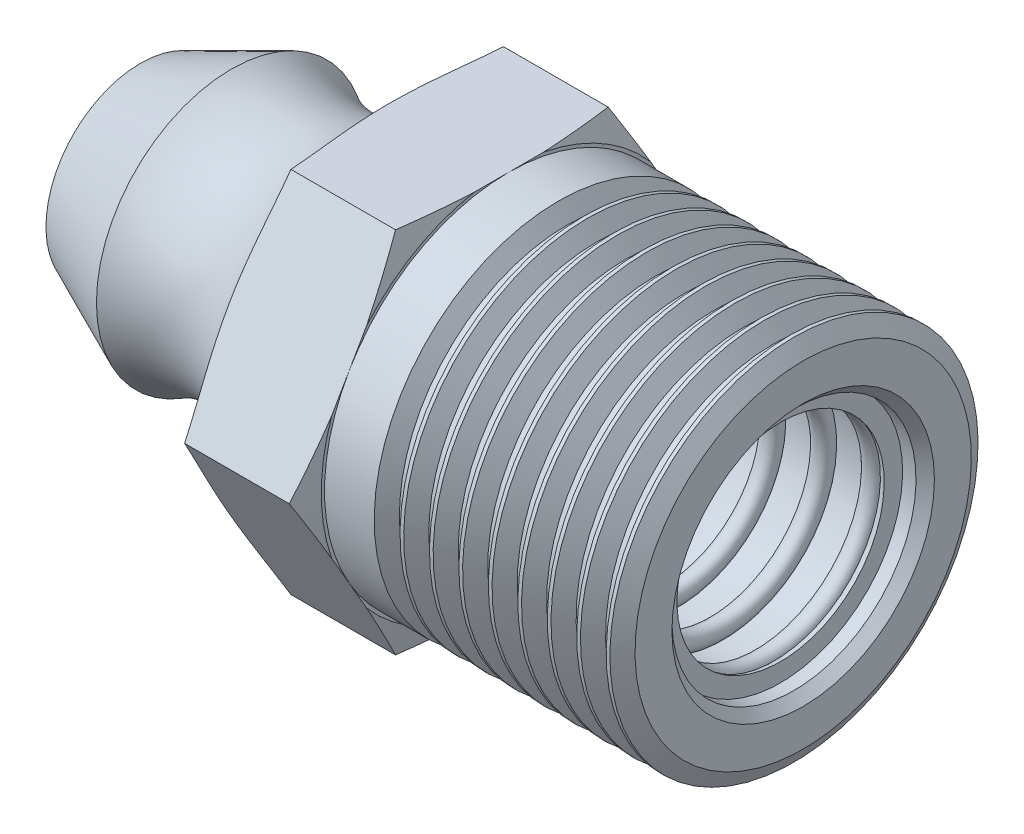
SolidWorks part; units mm, degrees
material "ASTM A36 钢"
ref_plane "前视基准面" through (0, 0, 0) normal (0, 0, 1) x (1, 0, 0)
ref_plane "上视基准面" through (0, 0, 0) normal (0, 1, 0) x (1, 0, 0)
ref_plane "右视基准面" through (0, 0, 0) normal (1, 0, 0) x (0, 0, -1)
sketch "草图1" plane through (0, 0, 0) normal (0, 0, 1) x (1, 0, 0)
  line L0 (-18.4, 0) -> (-15.9, 0)
  line L1 (-8, 5) -> (-8, 5.0885)
  line L2 (-11.5, 2.315) -> (-16.4719, 2.315)
  line L3 (-18, 1.0037) -> (-17.895, 1.0037)
  line L4 (-16.4719, 2.315) -> (-17.895, 1.0037)
  line L5 (-18, 2.565) -> (-15.5294, 3.665)
  line L6 (-0.25, 3.315) -> (-0.6135, 3.315)
  line L7 (-18, 2.565) -> (-18, 1.0037)
  line L8 (-11, 6.0885) -> (-8.2679, 6.0885)
  line L9 (-0.6135, 3.315) -> (-0.6135, 2.815)
  line L11 (-8, 5.0885) -> (-8.2679, 6.0885)
  line L12 (-10.5, 3.315) -> (-11.5, 2.315)
  line L13 (0, 3.565) -> (-0.25, 3.315)
  line L14 (-1.1135, 3.315) -> (-10.5, 3.315)
  line L68 (-6.2, 4.567) -> (-5.95, 5)
  line L69 (-3.2, 4.567) -> (-3, 4.567)
  line L71 (-5.6, 4.567) -> (-5.4, 4.567)
  line L72 (-5.15, 5) -> (-5.05, 5)
  line L73 (-4.35, 5) -> (-4.25, 5)
  line L78 (-6.4, 4.567) -> (-6.2, 4.567)
  line L79 (-5.85, 5) -> (-5.6, 4.567)
  line L80 (-0.8, 4.567) -> (-0.6, 4.567)
  line L81 (-0.25, 5) -> (0, 4.567)
  line L85 (-1.15, 5) -> (-1.05, 5)
  line L90 (-5.95, 5) -> (-5.85, 5)
  line L91 (-5.05, 5) -> (-4.8, 4.567)
  line L92 (-3.45, 5) -> (-3.2, 4.567)
  line L93 (-2.2, 4.567) -> (-1.95, 5)
  line L94 (-1.95, 5) -> (-1.85, 5)
  line L95 (-0.6, 4.567) -> (-0.35, 5)
  line L98 (-1.05, 5) -> (-0.8, 4.567)
  line L102 (-6.65, 5) -> (-6.4, 4.567)
  line L106 (-3.55, 5) -> (-3.45, 5)
  line L112 (-1.85, 5) -> (-1.6, 4.567)
  line L115 (-1.4, 4.567) -> (-1.15, 5)
  line L118 (-3.8, 4.567) -> (-3.55, 5)
  line L119 (-1.6, 4.567) -> (-1.4, 4.567)
  line L125 (-4.8, 4.567) -> (-4.6, 4.567)
  line L126 (-2.75, 5) -> (-2.65, 5)
  line L127 (-8, 5) -> (-6.65, 5)
  line L128 (-4, 4.567) -> (-3.8, 4.567)
  line L134 (-5.4, 4.567) -> (-5.15, 5)
  line L135 (-3, 4.567) -> (-2.75, 5)
  line L136 (-0.35, 5) -> (-0.25, 5)
  line L139 (-4.25, 5) -> (-4, 4.567)
  line L140 (-2.65, 5) -> (-2.4, 4.567)
  line L143 (-4.6, 4.567) -> (-4.35, 5)
  line L144 (-2.4, 4.567) -> (-2.2, 4.567)
  line L171 (0, 0) -> (-15.9, 0) construction
  line L178 (0, 4.567) -> (0, 3.565)
  circle A0 centre (-2.3502, 2.9066) radius 0.25
  arc A1 (-11, 6.0885) -> (-15.5294, 3.665) centre (-13.9601, 6.1764) cw
  arc A2 (-0.8635, 3.065) -> (-0.6135, 2.815) centre (-0.6135, 3.065) ccw
  arc A3 (-15.9, 0) -> (-18.4, 0) centre (-17.15, 0) ccw
  arc A4 (-0.8635, 3.065) -> (-1.1135, 3.315) centre (-1.1135, 3.065) ccw
  circle A5 centre (-1.1194, 3.0577) radius 0.25
  circle A6 centre (-3.581, 2.7555) radius 0.25
  circle A7 centre (-4.8117, 2.6043) radius 0.25
  circle A8 centre (-6.0425, 2.4532) radius 0.25
  circle A9 centre (-7.2732, 2.3021) radius 0.25
  circle A10 centre (-8.504, 2.151) radius 0.25
  circle A11 centre (-9.7347, 1.9999) radius 0.25
  circle A12 centre (-10.9655, 1.8488) radius 0.25
  circle A13 centre (-12.1963, 1.6976) radius 0.25
  circle A14 centre (-13.427, 1.5465) radius 0.25
  circle A15 centre (-14.6578, 1.3954) radius 0.25
  circle A16 centre (-15.8885, 1.2443) radius 0.25
  point P92 (-8, 6.0885)
  point P94 (-8, 6.0885)
  point P95 (0, 3.315)
  dimension "D4" = 45
  dimension "D5" = 5
  dimension "D6" = 0.5
  dimension "D8" = 1.25
  dimension "D9" = 0.35
  dimension "D1" = 1
  dimension "D7" = 2.9614
  dimension "D2" = 15
  dimension "D3" = 0.25
  dimension "D10" = 0.8
  dimension "D11" = 8
  dimension "D12" = 0.8635
  dimension "D13" = 1.2443
  dimension "D14" = 1.1194
  dimension "D15" = 1.3954
  dimension "D16" = 1.5465
  dimension "D17" = 1.6976
  dimension "D18" = 1.8488
  dimension "D19" = 1.9999
  dimension "D20" = 2.151
  dimension "D21" = 2.3502
  dimension "D22" = 2.3021
  dimension "D23" = 2.315
  dimension "D24" = 2.4532
  dimension "D25" = 2.565
  dimension "D26" = 2.6043
  dimension "D27" = 2.7555
  dimension "D28" = 2.815
  dimension "D29" = 3.581
  dimension "D30" = 2.9066
  dimension "D31" = 3.0577
  dimension "D32" = 3.665
  dimension "D36" = 4.8117
  dimension "D43" = 6.0425
  dimension "D47" = 7.2732
  dimension "D50" = 8.504
  dimension "D51" = 9.7347
  dimension "D52" = 10.5
  dimension "D53" = 10.9655
  dimension "D54" = 11
  dimension "D55" = 11.5
  dimension "D56" = 12.1963
  dimension "D57" = 13.427
  dimension "D58" = 13.9601
  dimension "D59" = 14.6578
  dimension "D60" = 15.5294
  dimension "D61" = 15.8885
  dimension "D62" = 16.4719
  dimension "D63" = 17.15
  dimension "D64" = 17.895
  dimension "D65" = 18
revolve "旋转1" add sketch "草图1" angle 360 about L171
sketch "草图2" plane through (0, 0, 0) normal (1, 0, 0) x (0, 0, -1)
  line L1 (5.7735, 0) -> (2.8868, 5)
  line L2 (2.8868, 5) -> (-2.8868, 5)
  line L3 (-2.8868, 5) -> (-5.7735, 0)
  line L4 (-5.7735, 0) -> (-2.8868, -5)
  line L5 (-2.8868, -5) -> (2.8868, -5)
  line L6 (2.8868, -5) -> (5.7735, 0)
  circle A0 centre (0, 0) radius 5 construction
  circle A1 centre (0, 0) radius 10.5391
  dimension "D2" = 21.0783
  dimension "D1" = 10
extrude "切除-拉伸1" cut sketch "草图2" against normal through all
